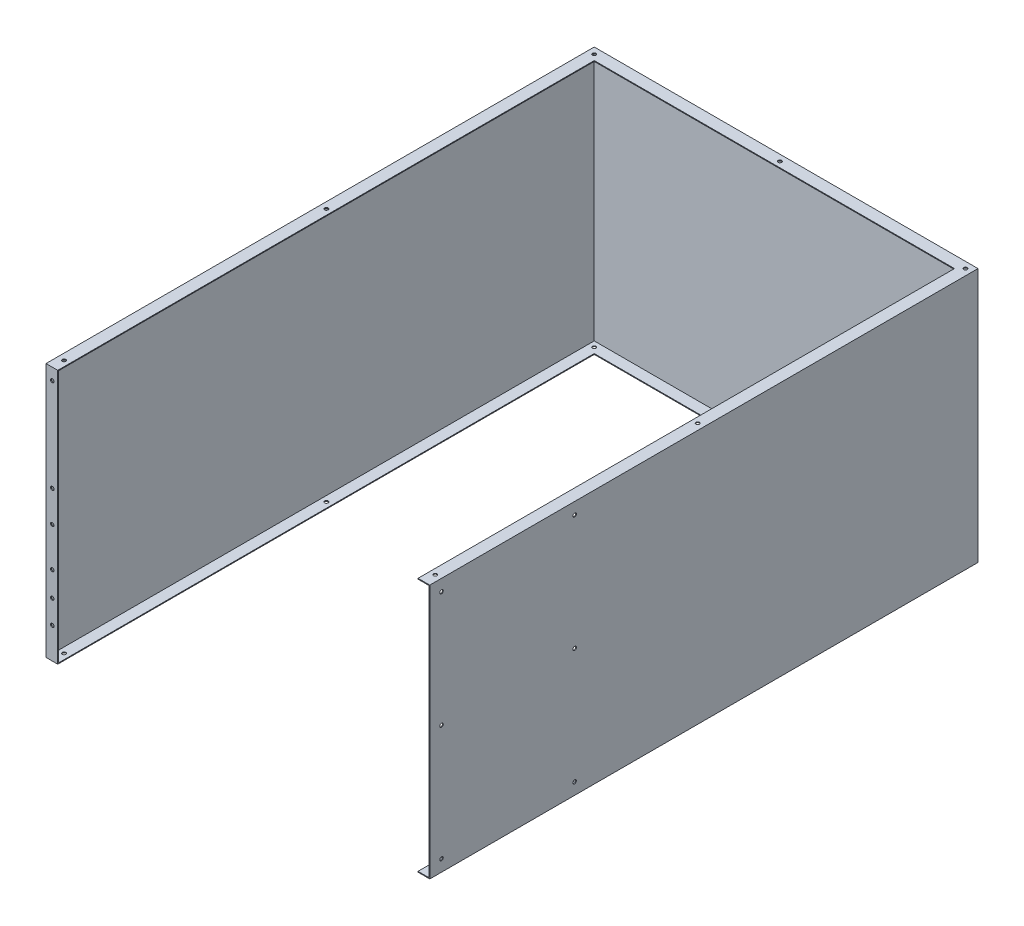
from build123d import *

# Parameters (mm, degrees)
EXTRUDE_1_DEPTH          = 325
EXTRUDE_2_DEPTH          = 2
EXTRUDE_3_DEPTH          = 2
SKETCH_5_W               = 30
SKETCH_5_H               = 650
EXTRUDE_4_DEPTH          = 2
SKETCH_6_R               = 4.5
CUT_EXTRUDE_1_DEPTH      = 10
CUT_EXTRUDE_2_DEPTH      = 1140
CUT_EXTRUDE_2_DEPTH_BACK = 345
SKETCH_7_R               = 4.5
SKETCH_8_R               = 4.5
CUT_EXTRUDE_3_DEPTH      = 10


with BuildPart() as part:
    # 草图1 → 凸台-拉伸1 (new, symmetric)
    with BuildSketch(Plane(origin=(0, 0, 0), x_dir=(1, 0, 0), z_dir=(0, 1, 0))):
        Polygon((-490, 700), (490, 700), (490, -700), (488, -700), (488, 698), (-488, 698), (-488, -700), (-490, -700), align=None)
    extrude(amount=EXTRUDE_1_DEPTH, both=True)

    # 草图2 → 凸台-拉伸2 (add)
    with BuildSketch(Plane(origin=(0, 325, 0), x_dir=(1, 0, 0), z_dir=(0, 1, 0))):
        Polygon((-490, 700), (-490, -700), (-460, -700), (-460, 670), (460, 670), (460, -700), (490, -700), (490, 700), align=None)
    extrude(amount=-EXTRUDE_2_DEPTH)

    # 草图3 → 凸台-拉伸3 (add)
    with BuildSketch(Plane.XZ.offset(325)):
        Polygon((490, -700), (490, 700), (460, 700), (460, -670), (-460, -670), (-460, 700), (-490, 700), (-490, -700), align=None)
    extrude(amount=-EXTRUDE_3_DEPTH)

    # 草图5 → 凸台-拉伸4 (add)
    with BuildSketch(Plane.XY.offset(700)):
        with Locations((-475, 0)):
            Rectangle(SKETCH_5_W, SKETCH_5_H)
    extrude(amount=-EXTRUDE_4_DEPTH)

    # 草图6 → 切除-拉伸1 (cut)
    with BuildSketch(Plane(origin=(0, 0, 698), x_dir=(-1, 0, 0), z_dir=(0, 0, -1))):
        with Locations((474, -246)):
            Circle(SKETCH_6_R)
        with Locations((474, -186)):
            Circle(SKETCH_6_R)
        with Locations((474, 295)):
            Circle(SKETCH_6_R)
        with Locations((474, 57)):
            Circle(SKETCH_6_R)
        with Locations((474, -23)):
            Circle(SKETCH_6_R)
        with Locations((474, -123)):
            Circle(SKETCH_6_R)
    extrude(amount=-CUT_EXTRUDE_1_DEPTH, mode=Mode.SUBTRACT)

    # 草图7 → 切除-拉伸2 (cut, two sides: drawn at the far end of the back side and taken through both)
    with BuildSketch(Plane.XZ.offset(-323).offset(-CUT_EXTRUDE_2_DEPTH_BACK)):
        with Locations(Location((-474, 670, 0), (0, 0, 90))):
            Circle(SKETCH_7_R)
        with Locations(Location((-474, 0, 0), (0, 0, 90))):
            Circle(SKETCH_7_R)
        with Locations(Location((-474, -684, 0), (0, 0, 90))):
            Circle(SKETCH_7_R)
        with Locations(Location((474, -684, 0), (0, 0, 90))):
            Circle(SKETCH_7_R)
        with Locations(Location((0, -684, 0), (0, 0, 90))):
            Circle(SKETCH_7_R)
        with Locations(Location((474, 0, 0), (0, 0, 90))):
            Circle(SKETCH_7_R)
        with Locations(Location((474, 670, 0), (0, 0, 90))):
            Circle(SKETCH_7_R)
    extrude(amount=CUT_EXTRUDE_2_DEPTH + CUT_EXTRUDE_2_DEPTH_BACK, mode=Mode.SUBTRACT)

    # 草图8 → 切除-拉伸3 (cut)
    with BuildSketch(Plane(origin=(490, 0, 0), x_dir=(0, 0, -1), z_dir=(1, 0, 0))):
        with Locations((-330, 295)):
            Circle(SKETCH_8_R)
        with Locations((-670, 295)):
            Circle(SKETCH_8_R)
        with Locations((-670, -295)):
            Circle(SKETCH_8_R)
        with Locations((-330, -295)):
            Circle(SKETCH_8_R)
        with Locations((-330, 0)):
            Circle(SKETCH_8_R)
        with Locations((-670, 0)):
            Circle(SKETCH_8_R)
    extrude(amount=-CUT_EXTRUDE_3_DEPTH, mode=Mode.SUBTRACT)


solid = part.part
